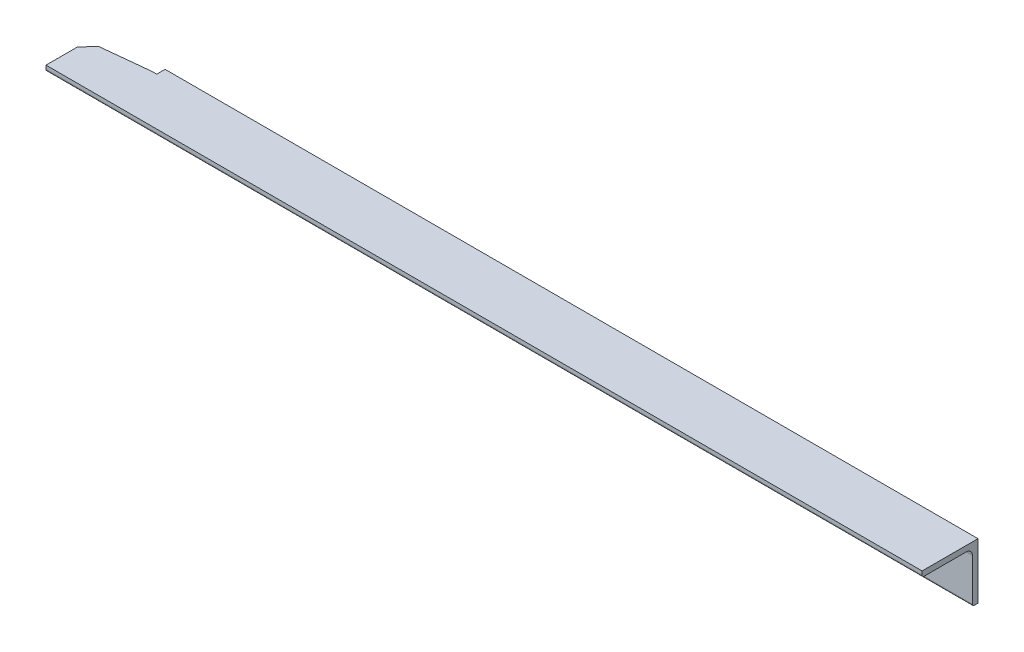
from build123d import *

# Parameters (mm, degrees)
GBT706_2008_050_5_1_DEPTH = 783.5
CUT_EXTRUDE_1_DEPTH       = 399.080472392
CUT_EXTRUDE_2_REACH       = 399.483


with BuildPart() as part:
    # Sketch1 → Gbt706-2008 热轧等边角钢 050×5(1) (new body)
    with BuildSketch(Plane(origin=(391.75, 0, 0), x_dir=(0, -1, 0), z_dir=(-1, 0, 0))):
        with BuildLine():
            Line((0, 0), (0, 50))
            Line((0, 50), (3.333333333, 50))
            ThreePointArc((3.333333333, 50), (4.511844635, 49.511844635), (5, 48.333333333))
            Line((5, 48.333333333), (5, 10.5))
            ThreePointArc((5, 10.5), (6.610912703, 6.610912703), (10.5, 5))
            Line((10.5, 5), (48.333333333, 5))
            ThreePointArc((48.333333333, 5), (49.511844635, 4.511844635), (50, 3.333333333))
            Line((50, 3.333333333), (50, 0))
            Line((50, 0), (0, 0))
        make_face()
    extrude(amount=GBT706_2008_050_5_1_DEPTH)

    # 草图2 → 切除-拉伸1 (cut, through all)
    with BuildSketch(Plane(origin=(0, 0, 0), x_dir=(1, 0, 0), z_dir=(0, 1, 0))):
        Polygon((-335.25, 0), (-335.25, -7.501394609), (-339.727357684, -7.501394609), (-382.795284633, -12.028016136), (-391.75, -21.973235089), (-391.75, -52.501394609), (-406.75, -52.501394609), (-406.75, 7.498605391), (-335.25, 7.498605391), align=None)
    extrude(amount=-CUT_EXTRUDE_1_DEPTH, mode=Mode.SUBTRACT)

    # 草图3 → 切除-拉伸2 (cut, up to next)
    with BuildSketch(Plane.XY.offset(5), mode=Mode.PRIVATE) as cut_extrude_2_sk1:
        with BuildLine():
            Line((-25.75, -25.5), (-21.75, -25.5))
            ThreePointArc((-21.75, -25.5), (-17.25, -30), (-21.75, -34.5))
            Line((-21.75, -34.5), (-25.75, -34.5))
            ThreePointArc((-25.75, -34.5), (-30.25, -30), (-25.75, -25.5))
        make_face()
    cut_extrude_2_tool1 = extrude(cut_extrude_2_sk1.sketch, amount=-CUT_EXTRUDE_2_REACH, mode=Mode.PRIVATE) & part.part
    # 草图3 → 切除-拉伸2 (cut, up to next)
    with BuildSketch(Plane.XY.offset(5), mode=Mode.PRIVATE) as cut_extrude_2_sk2:
        with BuildLine():
            Line((-311.75, -25.5), (-307.75, -25.5))
            ThreePointArc((-307.75, -25.5), (-303.25, -30), (-307.75, -34.5))
            Line((-307.75, -34.5), (-311.75, -34.5))
            ThreePointArc((-311.75, -34.5), (-316.25, -30), (-311.75, -25.5))
        make_face()
    cut_extrude_2_tool2 = extrude(cut_extrude_2_sk2.sketch, amount=-CUT_EXTRUDE_2_REACH, mode=Mode.PRIVATE) & part.part
    add(cut_extrude_2_tool1.solids().sort_by_distance((-23.75, -30, 5))[0], mode=Mode.SUBTRACT)
    add(cut_extrude_2_tool2.solids().sort_by_distance((-309.75, -30, 5))[0], mode=Mode.SUBTRACT)


solid = part.part
